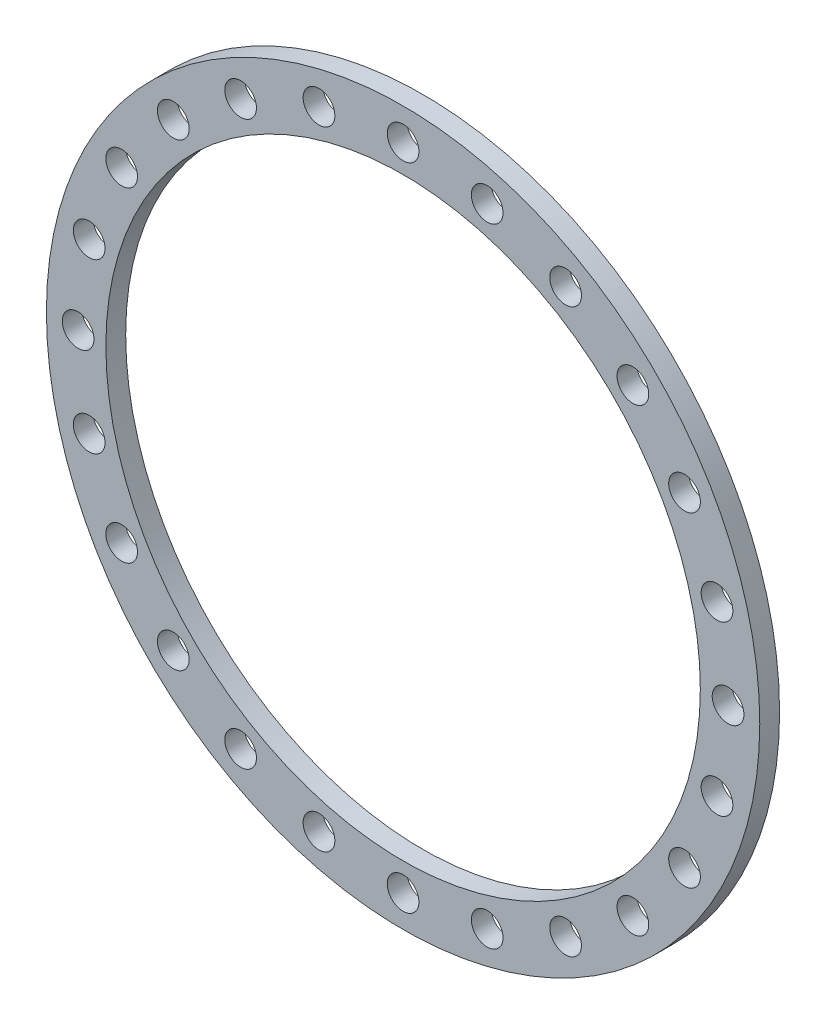
SolidWorks part; units mm, degrees
ref_plane "前视基准面" through (0, 0, 0) normal (0, 0, 1) x (1, 0, 0)
ref_plane "上视基准面" through (0, 0, 0) normal (0, 1, 0) x (1, 0, 0)
ref_plane "右视基准面" through (0, 0, 0) normal (1, 0, 0) x (0, 0, -1)
other "Configuration Table"
sketch "草图1" plane through (0, 0, 0) normal (0, 0, 1) x (1, 0, 0)
  circle A0 centre (0, 0) radius 450
  dimension "D1" = 900
extrude "凸台-拉伸1" add sketch "草图1" along normal blind 25 contours A0
sketch "草图2" plane through (0, 0, 25) normal (0, 0, 1) x (1, 0, 0)
  circle A0 centre (0, 0) radius 410 construction
  circle A1 centre (0, 410) radius 20
  circle A2 centre (106.1158, 396.0296) radius 20
  circle A3 centre (205, 355.0704) radius 20
  circle A4 centre (289.9138, 289.9138) radius 20
  circle A5 centre (355.0704, 205) radius 20
  circle A6 centre (396.0296, 106.1158) radius 20
  circle A7 centre (410, 0) radius 20
  circle A8 centre (396.0296, -106.1158) radius 20
  circle A9 centre (355.0704, -205) radius 20
  circle A10 centre (289.9138, -289.9138) radius 20
  circle A11 centre (205, -355.0704) radius 20
  circle A12 centre (106.1158, -396.0296) radius 20
  circle A13 centre (0, -410) radius 20
  circle A14 centre (-106.1158, -396.0296) radius 20
  circle A15 centre (-205, -355.0704) radius 20
  circle A16 centre (-289.9138, -289.9138) radius 20
  circle A17 centre (-355.0704, -205) radius 20
  circle A18 centre (-396.0296, -106.1158) radius 20
  circle A19 centre (-410, 0) radius 20
  circle A20 centre (-396.0296, 106.1158) radius 20
  circle A21 centre (-355.0704, 205) radius 20
  circle A22 centre (-289.9138, 289.9138) radius 20
  circle A23 centre (-205, 355.0704) radius 20
  circle A24 centre (-106.1158, 396.0296) radius 20
  dimension "D1" = 820
  dimension "D2" = 40
  dimension "D3" = 24
extrude "切除-拉伸1" cut sketch "草图2" against normal blind 34
sketch "草图3" plane through (0, 0, 25) normal (0, 0, 1) x (1, 0, 0)
  circle A0 centre (0, 0) radius 375
  dimension "D1" = 750
extrude "切除-拉伸2" cut sketch "草图3" against normal blind 420 contours A0
